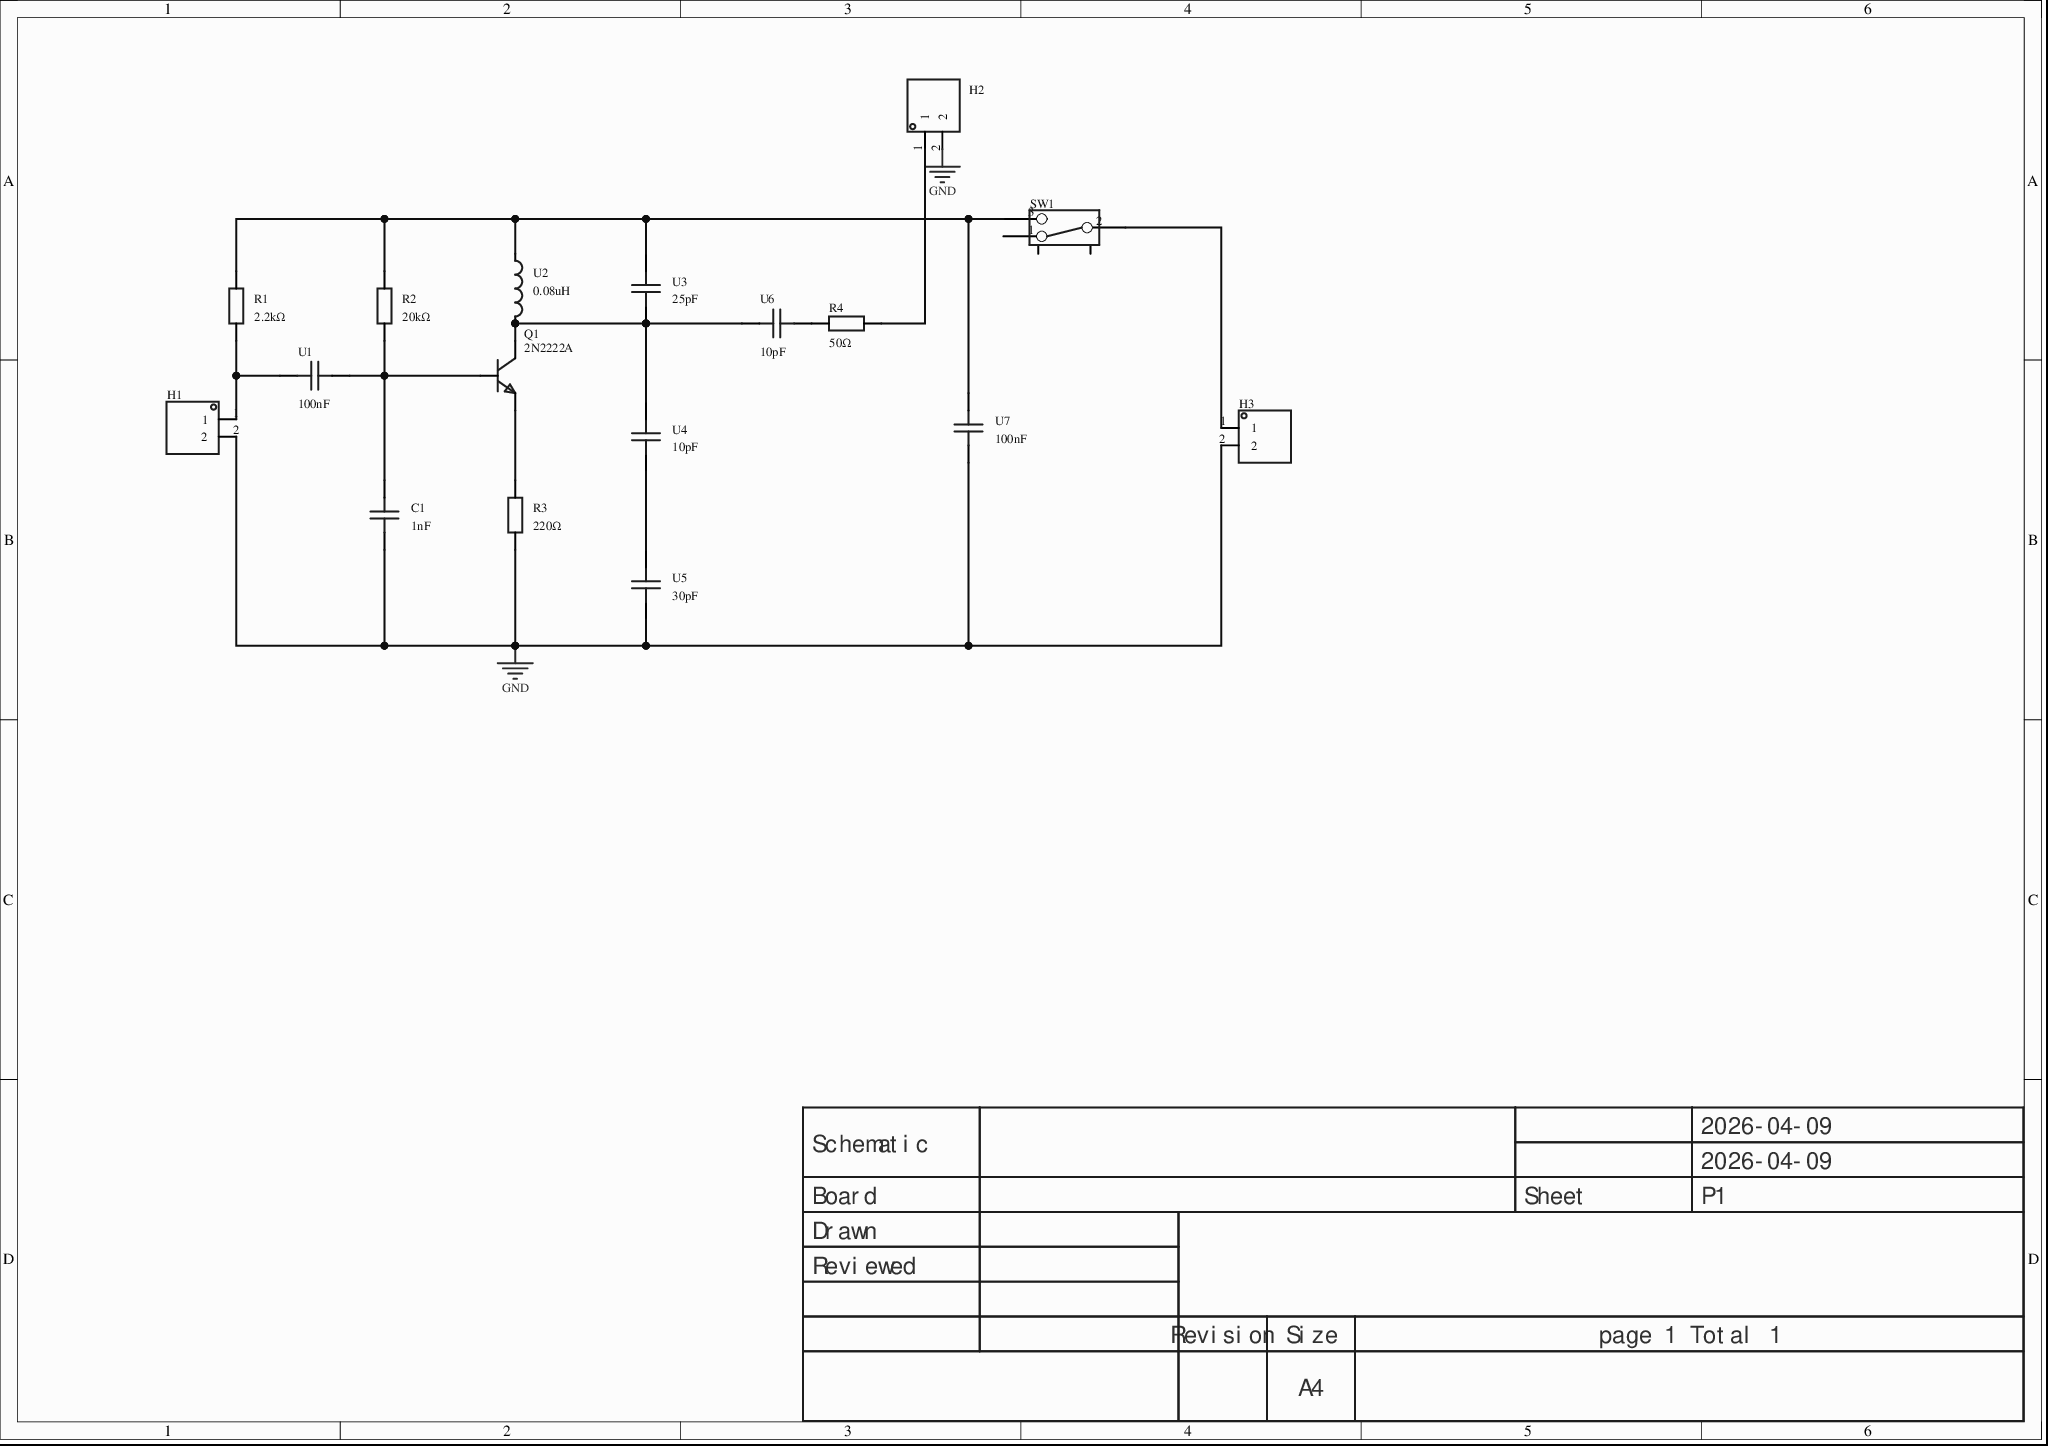
[diagram p0: MISC51145-3.schdoc]
# Altium project MISC51145-2.PrjPcb
1 sheet, 17 parts. Net scope: global (net labels, ports and power ports of the same name join across sheets).
Board file: MISC51145.pcbdoc

## Sheet MISC51145-3.schdoc
size 297 x 209 mm; Version: V1.0; @Project Name: MISC51145; @Update Date: 2026-04-09; @Create Date: 2026-04-09; @Board Name: MISC51145; @Create Time: 20:28:24; @Page Count: 1; @Page No: 1; @Schematic Name: MISC51145; @Update Time: 20:28:24; Size: A4

### Parts
C1  1nF  [CAP-TH_L7.0-W4.0-P10.00-D0.6-1]
H1  (no value)  [HDR-TH_2P-P2.54-V-M-1]
H2  (no value)  [HDR-TH_2P-P2.54-V-M-1]
H3  (no value)  [HDR-TH_2P-P2.54-V-M-1]
Q1  2N2222A  [TO-92-3_L5.1-W4.1-P1.27-L-1]
R1  2.2kΩ  [Res_1/8W]
R2  20kΩ  [Res_1/8W]
R3  220Ω  [Res_1/8W]
R4  50Ω  [Res_1/8W]
SW1  (no value)  [拨动开关_侧]
U1  100nF  [CAP-TH_L5.0-W2.5-P5.00-D1.0]
U2  0.08uH  [IND-TH_BD6.5-W9.2-LS14.0-D0.8]
U3  25pF  [CAP-TH_L5.0-W2.5-P5.00-D1.0]
U4  10pF  [CAP-TH_L5.0-W2.5-P5.00-D1.0]
U5  30pF  [CAP-TH_L5.0-W2.5-P5.00-D1.0]
U6  10pF  [CAP-TH_L5.0-W2.5-P5.00-D1.0]
U7  100nF  [CAP-TH_L5.0-W2.5-P5.00-D1.0]

### Nets
GND: C1.1 H1.2 H2.2 H3.2 R3.1 U5.2 U7.2
NetC1_2: C1.2 Q1.2(B) R2.1 U1.1
NetH1_1: H1.1 R1.1 U1.2
NetH2_1: H2.1 R4.2
NetH3_1: H3.1 SW1.2
NetQ1_1: Q1.1(E) R3.2
NetQ1_3: Q1.3(C) U2.2 U3.2 U4.1 U6.1
NetR1_2: R1.2 R2.2 SW1.3 U2.1 U3.1 U7.1
NetR4_1: R4.1 U6.2
NetU4_2: U4.2 U5.1

Not connected (* = marked no-connect by the designer): SW1 1 4 5

### Notes on the sheet
- 2026-04-09
- Schematic
- Board
- Sheet
- P1
- Drawn
- Reviewed
- Revision
- Size
- A4
- page 1 Total 1

### Library data of the parts
C1 = DE1E3RA102MJ4BH01F: Capacitance: 1nF; Tolerance: ±20%; Working voltage (AC): 400V; 440V; Protection class: X1,Y1;; Manufacturer: muRata(村田); AddInBom: yes; ModelId: c7b61f91d1404f65abb2cfc380a081b00819f05c4eef4c71ace90d822a990e87; ModelTransform: 437.12968,177.138,0,0,0,0,0,0,-137.795; Ratings: X1,Y1; Symbol: DE1E3RA102MJ4BH01F; Device: DE1E3RA102MJ4BH01F; LCSC Part Name: 1nF ±20% 440V 400V 等级:X1,Y1; SupplierPart: C6601326; ManufacturerPart: DE1E3RA102MJ4BH01F; Supplier Footprint: 插件,P=10mm; JLCPCB Part Class: Extended Part; Datasheet: https://item.szlcsc.com/datasheet/DE1E3RA102MJ4BH01F/7556258.html; Supplier: LCSC; ConvertToPcb: yes; FootprintName: CAP-TH_L7.0-W4.0-P10.00-D0.6-1; ModelName: CAP-TH_L7.0-W4.0-P10.00-D0.6-1; Value: 1nF; Voltage(AC): 400V; 440V; Operating Temperature: -40℃~+125℃
H1-H3 = HDR-M_2.54_1x2P: Symbol: 210S-1*2P L=11.6MMGold-plated black; ConvertToPcb: yes; ModelId: 79b2e9f2d70a4d68a1b7098f27c6d4c50819f05c4eef4c71ace90d822a990e87; ModelName: HDR-M-2.54_1x2; ModelTransform: 200,100,0,0,0,0,0,0,-118.11; Device: HDR-M_2.54_1x2P; AddInBom: yes; SupplierPart: C124375; Supplier Footprint: 插件; FootprintName: HDR-TH_2P-P2.54-V-M-1
Q1 = 2N2222A_C50229645: Transistor type: NPN.  Collector current ICM: 800MA  Collector-base breakdown voltage BVCBO: 60V  Collector-emitter breakdown voltage BVCEO: 30V  DC current gain HFE: 100-200; Manufacturer: DDF(鼎德丰); AddInBom: yes; ModelId: 3974197e164648709a3727be714795da0819f05c4eef4c71ace90d822a990e87; ModelTransform: 200.42283,161.417,0,0,0,0,0,9.842,-196.85; Symbol: 2N2222A_C50229645; Device: 2N2222A_C50229645; LCSC Part Name: 2N2222A; SupplierPart: C50229645; ManufacturerPart: 2N2222A; Supplier Footprint: TO-92; JLCPCB Part Class: Extended Part; Datasheet: https://item.szlcsc.com/datasheet/2N2222A/52814798.html; Supplier: LCSC; ConvertToPcb: yes; FootprintName: TO-92-3_L5.1-W4.1-P1.27-L-1; ModelName: TO-92-3_L5.1-W4.1-P1.27-L-1
R1-R4 = Res_AXIAL-1/8W: Symbol: Resistor; ConvertToPcb: yes; ModelId: b2b5ae7ae4c642178fe0039925c86a3f0819f05c4eef4c71ace90d822a990e87; ModelName: RES-TH_BD1.8-L3.2-P7.20-D0.4; ModelTransform: 282.86,66.88,253.09,0,0,0,0,0,-191; Device: Res_AXIAL-1/8W; AddInBom: yes; Supplier Footprint: 轴向引线; FootprintName: Res_1/8W
  R1: Value: 2.2kΩ
  R2: Value: 20kΩ
  R3: Value: 220Ω
  R4: Value: 50Ω
SW1 = 拨动开关_侧: Symbol: Toggle switch; Device: Toggle switch_side; ConvertToPcb: yes; ModelId: 10ea2cc5ba004a75b38812aadef1031f0819f05c4eef4c71ace90d822a990e87; ModelName: SW-TH_SK-12D07-VG3; ModelTransform: 337.98,287.46,295.24,0,0,0,0,-57,-110; AddInBom: yes; Supplier Footprint: 插件; FootprintName: Toggle switch_side
U1 U3-U7 = 100nF: Symbol: 100NF_C9900015256; AddInBom: yes; ModelId: 08e3d7481fc7486bb1b263873f51e1e10819f05c4eef4c71ace90d822a990e87; ModelName: CAP-TH_BD5.0-W2.5-P5.08; ModelTransform: 224.652,98.425,0,0,0,0,-0.005,0,-137.795; Device: 100nF; LCSC Part Name: 100nF; SupplierPart: C9900015256; Supplier Footprint: CAP-TH_L5.0-W2.5-P5.00-D1.0; JLCPCB Part Class: Extended Part; Supplier: LCSC; ConvertToPcb: yes; FootprintName: CAP-TH_L5.0-W2.5-P5.00-D1.0
  U1 U7: ManufacturerPart: 100nF
  U3: Manufacturer Part: 25pF
  U4 U6: Manufacturer Part: 10pF
  U5: Manufacturer Part: 30pF
U2 = B82144F2102K000: Inductance: 1uH; Tolerance: ±10%; Rated current: 4.45A; Saturation current (Isat): 7.7A; Type: color-band inductor; Quality factor: 50@2.52MHz;; Manufacturer: TDK; AddInBom: yes; ModelId: 03646ffa8850423188af3ae38f0992a80819f05c4eef4c71ace90d822a990e87; ModelTransform: 582.676,255.905,0,0,0,0,0,0,-196.85; DC Resistance(DCR): 43mΩ; Frequency - Self Resonant: 200MHz; Symbol: B82144F2102K000; Device: B82144F2102K000; Value: 0.08uH; LCSC Part Name: B82144F2102K000; ManufacturerPart: B82144F2102K000; Supplier Footprint: 插件,D6.5xL9.2mm; JLCPCB Part Class: Extended Part; Datasheet: https://item.szlcsc.com/datasheet/B82144F2102K000/2134639.html; Supplier: LCSC; ConvertToPcb: yes; FootprintName: IND-TH_BD6.5-W9.2-LS14.0-D0.8; ModelName: IND-TH_BD6.5-W9.2-LS14.0-D0.8; Current Rating: 4.45A; Current - Saturation(Isat): 7.7A; Type: Color-band inductor; Q @ Frequency: 50@2.52MHz; Ratings: -